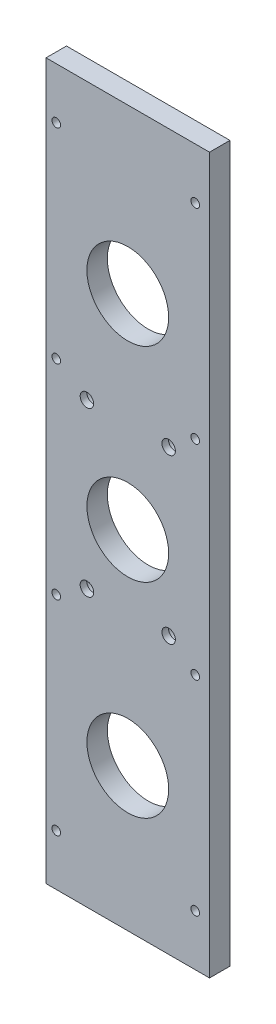
SolidWorks part; units mm, degrees
ref_plane "前视基准面" through (0, 0, 0) normal (0, 0, 1) x (1, 0, 0)
ref_plane "上视基准面" through (0, 0, 0) normal (0, 1, 0) x (1, 0, 0)
ref_plane "右视基准面" through (0, 0, 0) normal (1, 0, 0) x (0, 0, -1)
sketch "草图1" plane through (0, 0, 0) normal (0, 0, 1) x (1, 0, 0)
  line L1 (40, -175) -> (-40, -175)
  line L2 (40, -175) -> (40, 175)
  line L3 (40, 175) -> (-40, 175)
  line L4 (-40, -175) -> (-40, 175)
  line L5 (40, -175) -> (-40, 175) construction
  line L6 (40, 175) -> (-40, -175) construction
  point P0 (0, 0)
  dimension "D1" = 80
  dimension "D2" = 350
extrude "凸台-拉伸1" add sketch "草图1" along normal blind 10
hole_wizard "M5 螺纹孔1" positions "草图2" profile "草图3" tap size "M5" standard "GB" end condition up to next
sketch "草图2" plane through (0, 0, 0) normal (0, 0, -1) x (-1, 0, 0)
  point P0 (-33, 150)
  point P3 (35, 150)
  point P6 (-33, 50)
  point P9 (35, 50)
  point P12 (-33, -50)
  point P15 (35, -50)
  point P18 (-33, -150)
  point P21 (35, -150)
sketch "草图3" plane through (33, 150, 0) normal (1, 0, 0) x (0, 1, 0)
  line L0 (0, 0) -> (0, 10)
  line L1 (0, 10) -> (2.1, 10)
  line L2 (2.1, 10) -> (2.1, 0)
  line L5 (2.1, 0) -> (0, 0)
  line L11 (0, -6.35) -> (0, 107.95) construction
  dimension "通孔螺纹孔钻头直径" = 4.2
  dimension "通孔螺纹孔钻头深度" = 10
cosmetic thread "孔螺蚊线1" parameters "D2"=5
cosmetic thread "孔螺蚊线2" parameters "D2"=5
cosmetic thread "孔螺蚊线3" parameters "D2"=5
cosmetic thread "孔螺蚊线4" parameters "D2"=5
cosmetic thread "孔螺蚊线5" parameters "D2"=5
cosmetic thread "孔螺蚊线6" parameters "D2"=5
cosmetic thread "孔螺蚊线7" parameters "D2"=5
cosmetic thread "孔螺蚊线8" parameters "D2"=5
hole_wizard "打孔尺寸(%根据)内六角圆柱头螺钉的类型1" positions "草图4" profile "草图5" counterbore size "M6" standard "GB" end condition up to next
sketch "草图4" plane through (0, 0, 0) normal (0, 0, -1) x (-1, 0, 0)
  point P0 (-20, 40)
  point P2 (20, 40)
  point P5 (20, -40)
  point P8 (-20, -40)
sketch "草图5" plane through (20, 40, 0) normal (1, 0, 0) x (0, 1, 0)
  line L0 (0, 0) -> (0, 10)
  line L1 (0, 10) -> (3.3, 10)
  line L3 (3.3, 10) -> (3.3, 6.8)
  line L4 (3.3, 6.8) -> (5.5, 6.8)
  line L5 (5.5, 6.8) -> (5.5, 0)
  line L7 (5.5, 0) -> (0, 0)
  line L11 (0, -6.35) -> (0, 107.95) construction
  dimension "通孔孔直径" = 6.6
  dimension "通孔孔深度" = 10
  dimension "柱形沉头孔直径" = 11
  dimension "柱形沉头孔深度" = 6.8
sketch "草图6" plane through (0, 0, 0) normal (0, 0, -1) x (-1, 0, 0)
  line L0 (0, -175) -> (0, -105) construction
  line L1 (40, -175) -> (-40, -175) construction
  circle A0 centre (0, -105) radius 20
  dimension "D1" = 40
  dimension "D2" = 70
extrude "切除-拉伸1" cut sketch "草图6" against normal up to next
pattern_linear "阵列(线性)1" count 3 spacing 100 along (0, 1, 0) of "切除-拉伸1"
